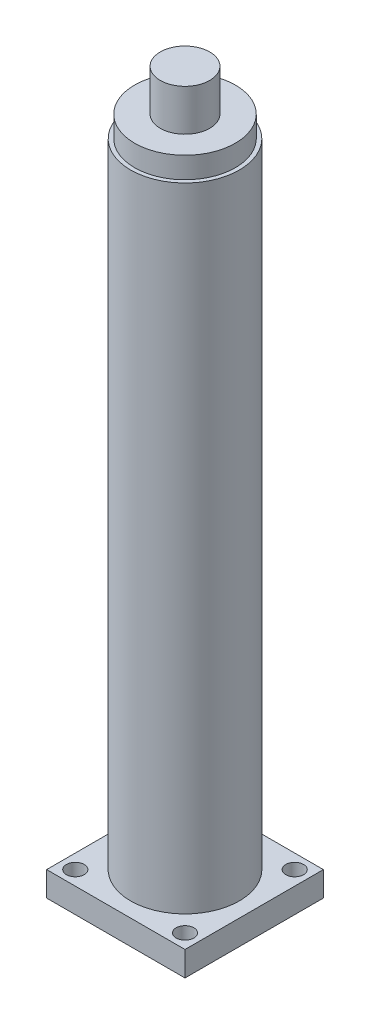
from build123d import *

# Parameters (mm, degrees)
SKETCH2_W           = 140
SKETCH2_H           = 140
SKETCH2_R           = 9
BOSS_EXTRUDE1_DEPTH = 25


with BuildPart() as part:
    # Sketch1 → Revolve1 (revolve)
    with BuildSketch(Plane.XY, mode=Mode.PRIVATE) as revolve1_sk:
        Polygon((0, 0), (60, 0), (60, 25), (55, 25), (55, 665.5), (51, 665.5), (51, 687), (25, 687), (25, 729), (0, 729), align=None)
    revolve(revolve1_sk.sketch.rotate(Axis((0, 0, 0), (0, -1, 0)), 90), axis=Axis((0, 0, 0), (0, -1, 0)))

    # Sketch2 → Boss-Extrude1 (add)
    with BuildSketch(Plane(origin=(0, 0, 0), x_dir=(1, 0, 0), z_dir=(0, 1, 0))):
        Rectangle(SKETCH2_W, SKETCH2_H)
        with Locations(Location((-55.5, 55.5, 0), (0, 0, 270))):
            Circle(SKETCH2_R, mode=Mode.SUBTRACT)
        with Locations(Location((55.5, 55.5, 0), (0, 0, 270))):
            Circle(SKETCH2_R, mode=Mode.SUBTRACT)
        with Locations(Location((55.5, -55.5, 0), (0, 0, 270))):
            Circle(SKETCH2_R, mode=Mode.SUBTRACT)
        with Locations(Location((-55.5, -55.5, 0), (0, 0, 270))):
            Circle(SKETCH2_R, mode=Mode.SUBTRACT)
    extrude(amount=BOSS_EXTRUDE1_DEPTH)


solid = part.part
